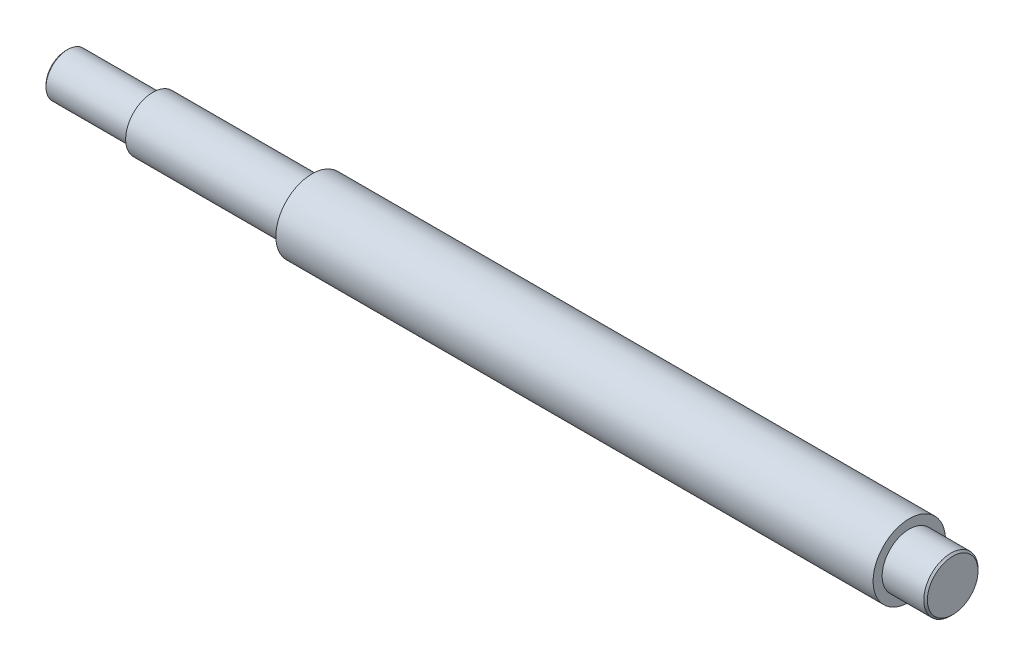
SolidWorks part; units mm, degrees
material "标准件"
ref_plane "前视基准面" through (0, 0, 0) normal (0, 0, 1) x (1, 0, 0)
ref_plane "上视基准面" through (0, 0, 0) normal (0, 1, 0) x (1, 0, 0)
ref_plane "右视基准面" through (0, 0, 0) normal (1, 0, 0) x (0, 0, -1)
sketch "草图1" plane through (0, 0, 0) normal (0, 1, 0) x (1, 0, 0)
  line L0 (0, 0) -> (245, 0) construction
  line L1 (0, 0) -> (0, 6)
  line L2 (0, 6) -> (24, 6)
  line L3 (24, 6) -> (24, 7.5)
  line L4 (24, 7.5) -> (68, 7.5)
  line L5 (68, 7.5) -> (68, 10)
  line L6 (68, 10) -> (233, 10)
  line L7 (233, 10) -> (233, 7.5)
  line L8 (233, 7.5) -> (245, 7.5)
  line L9 (245, 7.5) -> (245, 0)
  line L10 (0, 0) -> (245, 0)
  dimension "D1" = 44
  dimension "D2" = 15
  dimension "D3" = 12
  dimension "D4" = 20
  dimension "D5" = 24
  dimension "D6" = 12
  dimension "D7" = 15
  dimension "D8" = 165
revolve "旋转1" add sketch "草图1" angle 360 about L0
cosmetic thread "装饰螺纹线1" parameters "D2"=17.294
cosmetic thread "装饰螺纹线2" parameters "D1"=10, "D2"=11.797
ref_plane "基准面1" through (0, -6, 0) normal (0, -1, 0) x (-1, 0, 0)
sketch "草图2" plane through (0, -6, 0) normal (0, -1, 0) x (-1, 0, 0)
  line L0 (-24, 0) -> (0, 0) construction
  line L1 (-24, -7.5) -> (-24, 7.5) construction
  line L2 (-21, 0) -> (-3, 0) construction
  line L3 (-21, 2) -> (-3, 2)
  line L4 (-21, -2) -> (-3, -2)
  line L5 (0, -6) -> (0, 6) construction
  arc A0 (-21, 2) -> (-21, -2) centre (-21, 0) ccw
  arc A1 (-3, -2) -> (-3, 2) centre (-3, 0) ccw
  point P7 (-12, 0)
  dimension "D1" = 4
  dimension "D2" = 1
extrude "切除-拉伸1" cut sketch "草图2" against normal blind 2.2
chamfer "倒角1" distance 0.5 angle 45 2 edges at (245, 0, 7.5) (0, 0, 6)
